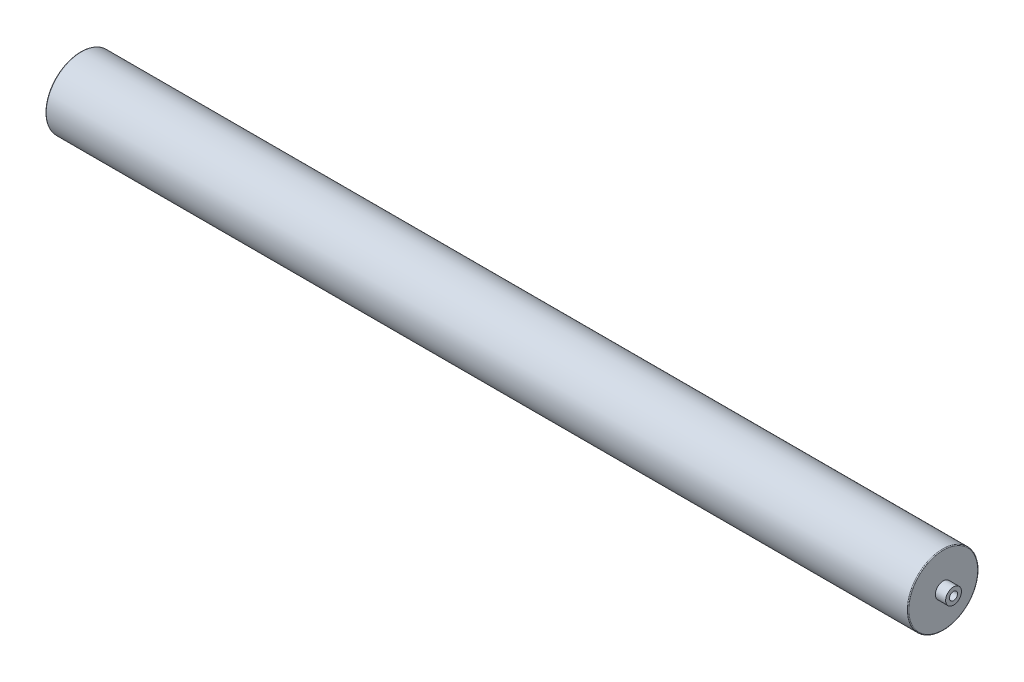
SolidWorks part; units mm, degrees
ref_plane "Front Plane" through (0, 0, 0) normal (0, 0, 1) x (1, 0, 0)
ref_plane "Top Plane" through (0, 0, 0) normal (0, 1, 0) x (1, 0, 0)
ref_plane "Right Plane" through (0, 0, 0) normal (1, 0, 0) x (0, 0, -1)
sketch "Sketch1" plane through (0, 0, 0) normal (1, 0, 0) x (0, 0, -1)
  circle A0 centre (0, 0) radius 44.5
  dimension "D1" = 89
extrude "Boss-Extrude1" add sketch "Sketch1" along normal mid plane 1090
sketch "Sketch2" plane through (545, 0, 0) normal (1, 0, 0) x (0, 0, -1)
  circle A0 centre (0, 0) radius 10
  dimension "D1" = 20
extrude "Boss-Extrude2" add sketch "Sketch2" along normal blind 13
sketch "Sketch3" plane through (-545, 0, 0) normal (-1, 0, 0) x (0, 0, 1)
  circle A0 centre (0, 0) radius 10
  dimension "D1" = 20
extrude "Boss-Extrude3" add sketch "Sketch3" along normal blind 13
fillet "Fillet1" radius 1 2 edges at (545, 0, -44.5) (-545, 0, -44.5)
hole_wizard "M12 Tapped Hole1" positions "3DSketch1" profile "Sketch4" tap size "M12" standard "GB"
sketch3d "3DSketch1"
  line L0 (558, 0, 0) -> (545, 0, 0) construction
  line L1 (-558, 0, 0) -> (-545, 0, 0) construction
  point P0 (558, 0, 0)
  point P4 (-558, 0, 0)
sketch "Sketch4" plane through (558, 0, 0) normal (0, 1, 0) x (0, 0, -1)
  line L0 (0, 0) -> (0, 23.0644)
  line L1 (0, 23.0644) -> (5.1, 20)
  line L2 (5.1, 20) -> (5.1, 0)
  line L5 (5.1, 0) -> (0, 0)
  line L10 (0, 23.0644) -> (-5.1, 20) construction
  line L11 (0, -6.35) -> (0, 107.95) construction
  dimension "螺纹孔钻头直径" = 10.2
  dimension "螺纹孔钻头深度" = 20
  dimension "导头角度" = 118
cosmetic thread "Hole thread1"
cosmetic thread "Hole thread2"
